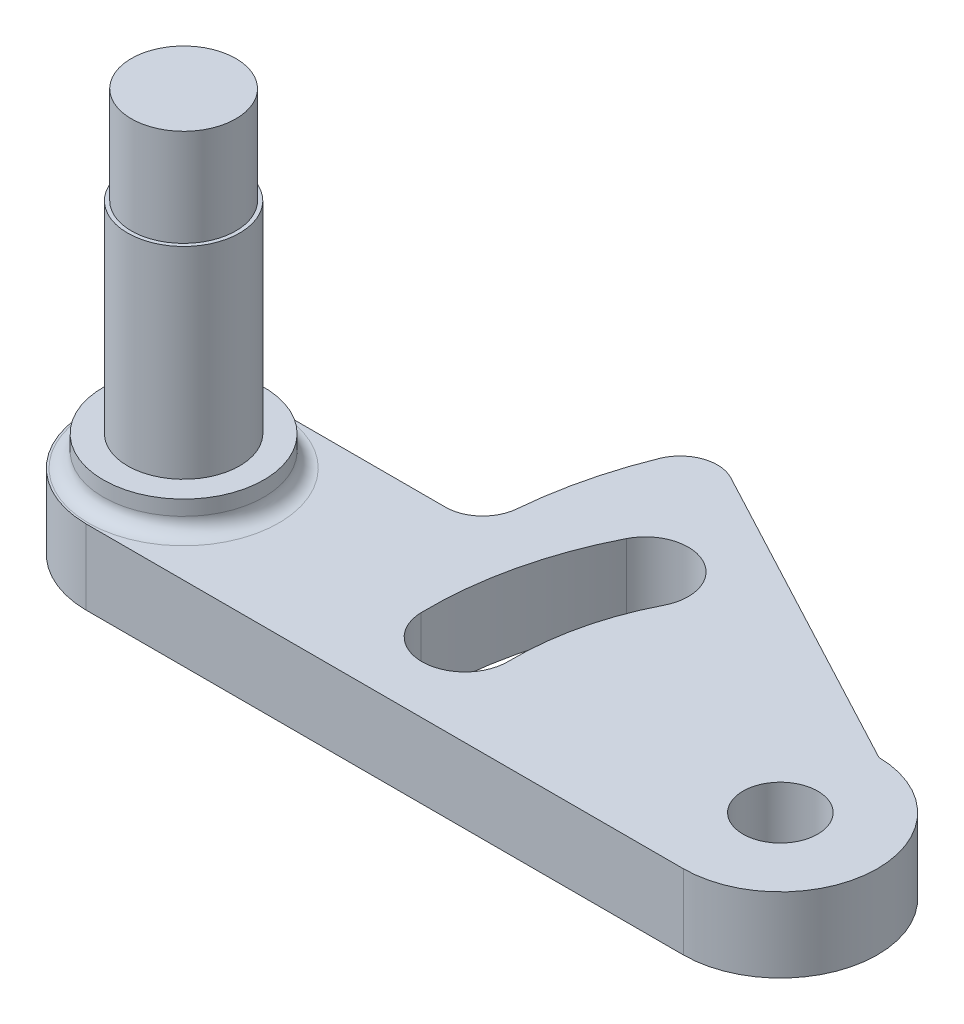
from build123d import *

# Parameters (mm, degrees)
SKETCH_1_R      = 5
EXTRUDE_1_DEPTH = 10
FILLET_2_R      = 5
SKETCH_2_R      = 10.75
EXTRUDE_2_DEPTH = 4
FILLET_3_R      = 2
SKETCH_3_R      = 7.5
EXTRUDE_3_DEPTH = 27
SKETCH_5_R      = 7
EXTRUDE_4_DEPTH = 13


with BuildPart() as part:
    # 草图1 → 凸台-拉伸1 (new body)
    with BuildSketch(Plane(origin=(0, 0, 0), x_dir=(1, 0, 0), z_dir=(0, 1, 0))):
        with BuildLine():
            Line((0, 0), (80, 0))
            ThreePointArc((80, 0), (92.999656788, 12.905536238), (80.188922536, 25.998627169))
            Line((80.188922536, 25.998627169), (33.171963216, 50.997987887))
            ThreePointArc((33.171963216, 50.997987887), (28.520841175, 38.881634135), (26.938922553, 26))
            Line((26.938922553, 26), (0.188922547, 26))
            ThreePointArc((0.188922547, 26), (-12.905538726, 13.094461274), (0, 0))
        make_face()
        with Locations(Location((80, 13, 0), (0, 0, 270))):
            Circle(SKETCH_1_R, mode=Mode.SUBTRACT)
        with BuildLine():
            ThreePointArc((48.162206807, 29.260917091), (45.167661271, 21.048023276), (44.255838588, 12.353915663))
            ThreePointArc((44.255838588, 12.353915663), (38.610693325, 6.500939074), (32.757716736, 12.146084337))
            ThreePointArc((32.757716736, 12.146084337), (33.962853008, 23.636897896), (37.920678927, 34.491701609))
            ThreePointArc((37.920678927, 34.491701609), (45.656835127, 36.99707329), (48.162206807, 29.260917091))
        make_face(mode=Mode.SUBTRACT)
    extrude(amount=EXTRUDE_1_DEPTH)

    # 圆角2
    fillet_2_edges = [part.edges().sort_by_distance(p)[0] for p in [
        (26.938922553, 5, -26),
        (33.171963216, 5, -50.997987887),
    ]]
    fillet(fillet_2_edges, radius=FILLET_2_R)

    # 草图2 → 凸台-拉伸2 (add)
    with BuildSketch(Plane(origin=(0, 10, 0), x_dir=(1, 0, 0), z_dir=(0, 1, 0))):
        with Locations(Location((0.094461274, 13, 0), (0, 0, 270))):
            Circle(SKETCH_2_R)
    extrude(amount=EXTRUDE_2_DEPTH)

    # 圆角3
    fillet_3_edges = [part.edges().sort_by_distance(p)[0] for p in [
        (0.094461274, 10, -23.75),
    ]]
    fillet(fillet_3_edges, radius=FILLET_3_R)

    # 草图3 → 凸台-拉伸3 (add)
    with BuildSketch(Plane(origin=(0, 14, 0), x_dir=(1, 0, 0), z_dir=(0, 1, 0))):
        with Locations(Location((0.094461274, 13, 0), (0, 0, 270))):
            Circle(SKETCH_3_R)
    extrude(amount=EXTRUDE_3_DEPTH)

    # 草图5 → 凸台-拉伸4 (add)
    with BuildSketch(Plane(origin=(0, 41, 0), x_dir=(1, 0, 0), z_dir=(0, 1, 0))):
        with Locations(Location((0.094461274, 13, 0), (0, 0, 90))):
            Circle(SKETCH_5_R)
    extrude(amount=EXTRUDE_4_DEPTH)


solid = part.part
